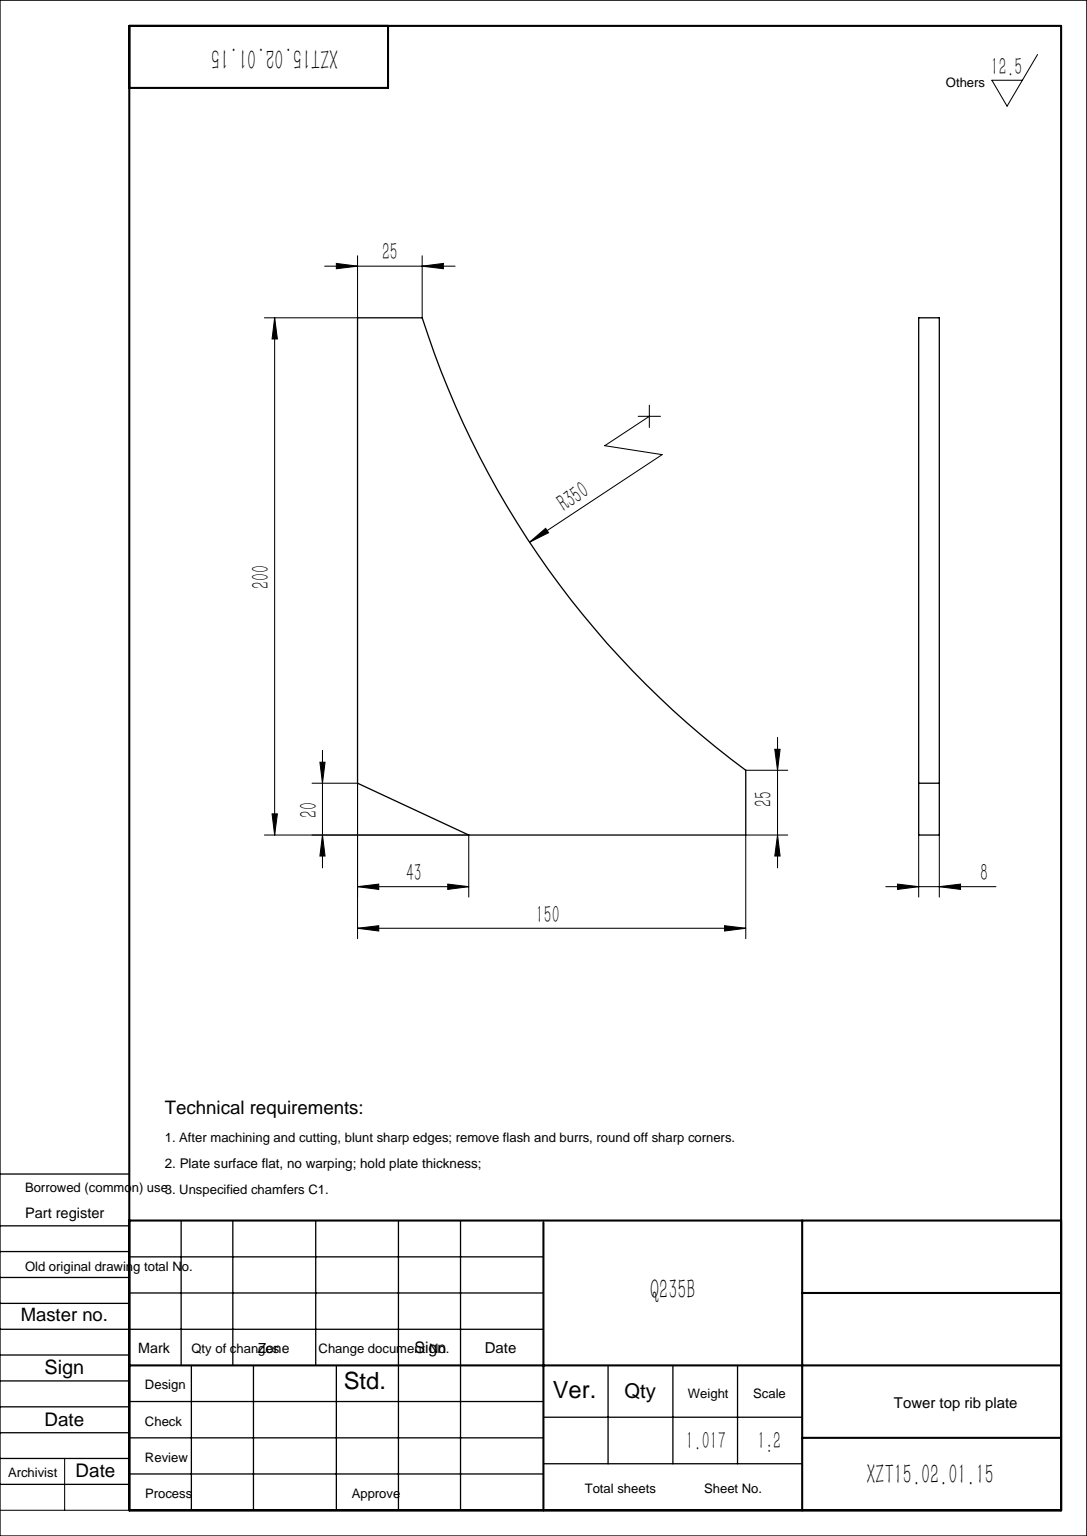
from build123d import *

# Parameters (mm, degrees)
BOSS_EXTRUDE1_DEPTH = 4
CHAMFER1_SIZE       = 20
CHAMFER1_SIZE2      = 43
CUT_EXTRUDE1_DEPTH  = 10


with BuildPart() as part:
    # Sketch1 → Boss-Extrude1 (new, symmetric)
    with BuildSketch(Plane.XY):
        Polygon((0, 0), (150, 0), (150, 25), (25, 200), (0, 200), align=None)
    extrude(amount=BOSS_EXTRUDE1_DEPTH, both=True)

    # Chamfer1
    chamfer1_edges = [part.edges().sort_by_distance(p)[0] for p in [
        (0, 0, 0),
    ]]
    chamfer1_side = [part.faces().sort_by_distance(p)[0] for p in [
        (0, 100, 0),
    ]]
    chamfer(chamfer1_edges, length=CHAMFER1_SIZE, length2=CHAMFER1_SIZE2, reference=chamfer1_side[0])

    # Sketch2 → Cut-Extrude1 (cut)
    with BuildSketch(Plane.XY.offset(4)):
        with BuildLine():
            ThreePointArc((25, 200), (73.72578288, 102.661273486), (150, 25))
            Line((150, 25), (25, 200))
        make_face()
    extrude(amount=-CUT_EXTRUDE1_DEPTH, mode=Mode.SUBTRACT)


solid = part.part
